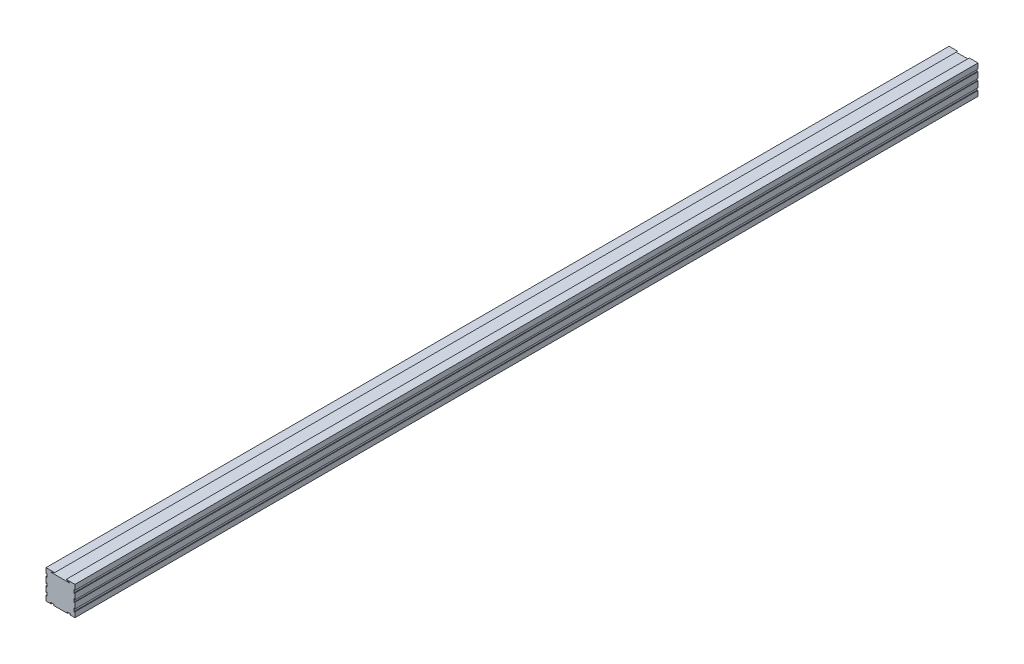
from build123d import *

# Parameters (mm, degrees)
SKETCH_1_W               = 75
SKETCH_1_H               = 75
EXTRUDE_1_DEPTH          = 1170
CUT_EXTRUDE_1_DEPTH      = 1170
CUT_EXTRUDE_2_DEPTH      = 2340
CUT_EXTRUDE_3_DEPTH      = 2341.600884388
CUT_EXTRUDE_3_DEPTH_BACK = 2341.600884388


with BuildPart() as part:
    # 草图1 → 凸台-拉伸1 (new, symmetric)
    with BuildSketch(Plane.XY):
        Rectangle(SKETCH_1_W, SKETCH_1_H)
    extrude(amount=EXTRUDE_1_DEPTH, both=True)

    # 草图2 → 切除-拉伸1 (cut, symmetric)
    with BuildSketch(Plane.XY):
        Polygon((-17.9, -36.8), (-16.55, -36.8), (-16.55, -34.5), (-25.45, -34.5), (-25.45, -36.8), (-24.1, -36.8), (-24.1, -37.5), (-17.9, -37.5), align=None)
        Polygon((16.55, -34.5), (16.55, -36.8), (17.9, -36.8), (17.9, -37.5), (24.1, -37.5), (24.1, -36.8), (25.45, -36.8), (25.45, -34.5), align=None)
    extrude(amount=CUT_EXTRUDE_1_DEPTH, both=True, mode=Mode.SUBTRACT)

    # 草图3 → 切除-拉伸2 (cut)
    with BuildSketch(Plane.XY.offset(1170)):
        Polygon((37.5, 2.6), (36.8, 2.6), (36.8, 4.45), (34.5, 4.45), (34.5, -4.45), (36.8, -4.45), (36.8, -2.6), (37.5, -2.6), align=None)
        Polygon((37.5, -17.9), (36.8, -17.9), (36.8, -16.55), (34.5, -16.55), (34.5, -25.45), (36.8, -25.45), (36.8, -24.1), (37.5, -24.1), align=None)
        Polygon((36.8, 24.1), (36.8, 25.45), (34.5, 25.45), (34.5, 16.55), (36.8, 16.55), (36.8, 17.9), (37.5, 17.9), (37.5, 24.1), align=None)
    cut_extrude_2 = extrude(amount=-CUT_EXTRUDE_2_DEPTH, mode=Mode.SUBTRACT)

    # 镜向1: 切除-拉伸2 across plane
    add(cut_extrude_2.mirror(Plane(origin=(0, 0, 0), x_dir=(0, 0, 1), z_dir=(1, 0, 0))), mode=Mode.SUBTRACT)

    # 草图4 → 切除-拉伸3 (cut, two sides: drawn at the far end of the back side and taken through both)
    with BuildSketch(Plane.XY.offset(1170).offset(-CUT_EXTRUDE_3_DEPTH_BACK)):
        Polygon((164.287302387, 109.214920955), (-15, 37.5), (-25, 33.5), (25, 33.5), (15, 37.5), (-164.287302387, 109.214920955), (-164.287302387, -276.981747517), (164.287302387, -276.981747517), align=None)
    extrude(amount=CUT_EXTRUDE_3_DEPTH + CUT_EXTRUDE_3_DEPTH_BACK, mode=Mode.SUBTRACT)


solid = part.part
